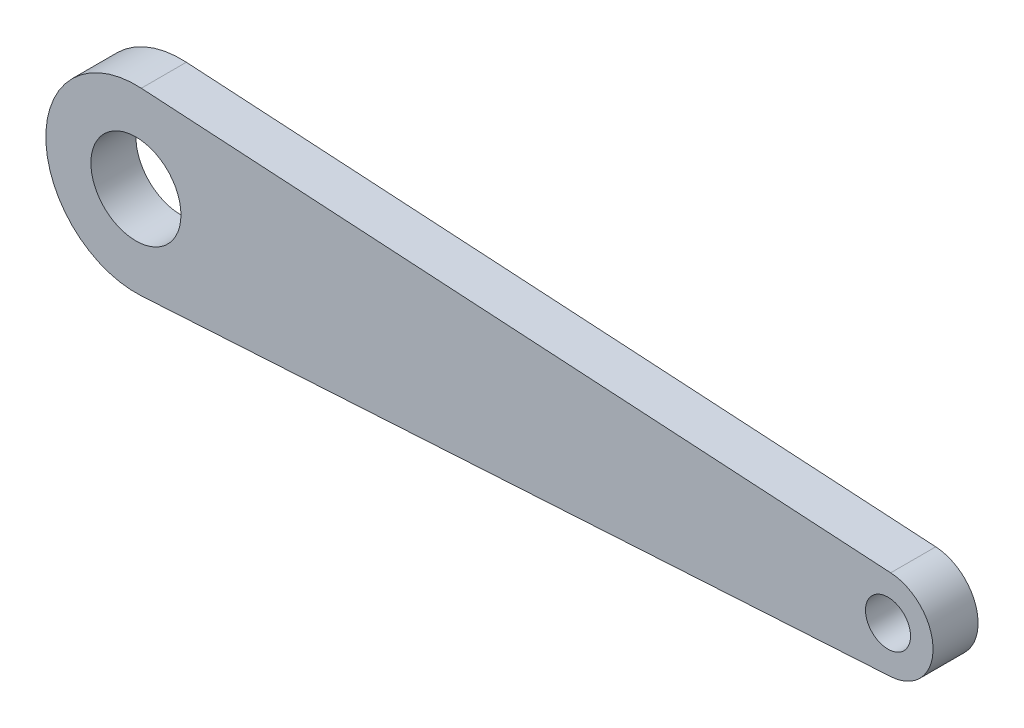
from build123d import *

# Parameters (mm, degrees)
SKETCH1_R           = 100
SKETCH1_R_2         = 50
BOSS_EXTRUDE1_DEPTH = 100


with BuildPart() as part:
    # Sketch1 → Boss-Extrude1 (new body)
    with BuildSketch(Plane.XY):
        with BuildLine():
            Line((11.976047904, 199.641113693), (1675.988023952, 99.820556847))
            ThreePointArc((1675.988023952, 99.820556847), (1770, 0), (1675.988023952, -99.820556847))
            Line((1675.988023952, -99.820556847), (11.976047904, -199.641113693))
            ThreePointArc((11.976047904, -199.641113693), (-200, 0), (11.976047904, 199.641113693))
        make_face()
        Circle(SKETCH1_R, mode=Mode.SUBTRACT)
        with Locations((1670, 0)):
            Circle(SKETCH1_R_2, mode=Mode.SUBTRACT)
    extrude(amount=BOSS_EXTRUDE1_DEPTH)


solid = part.part
